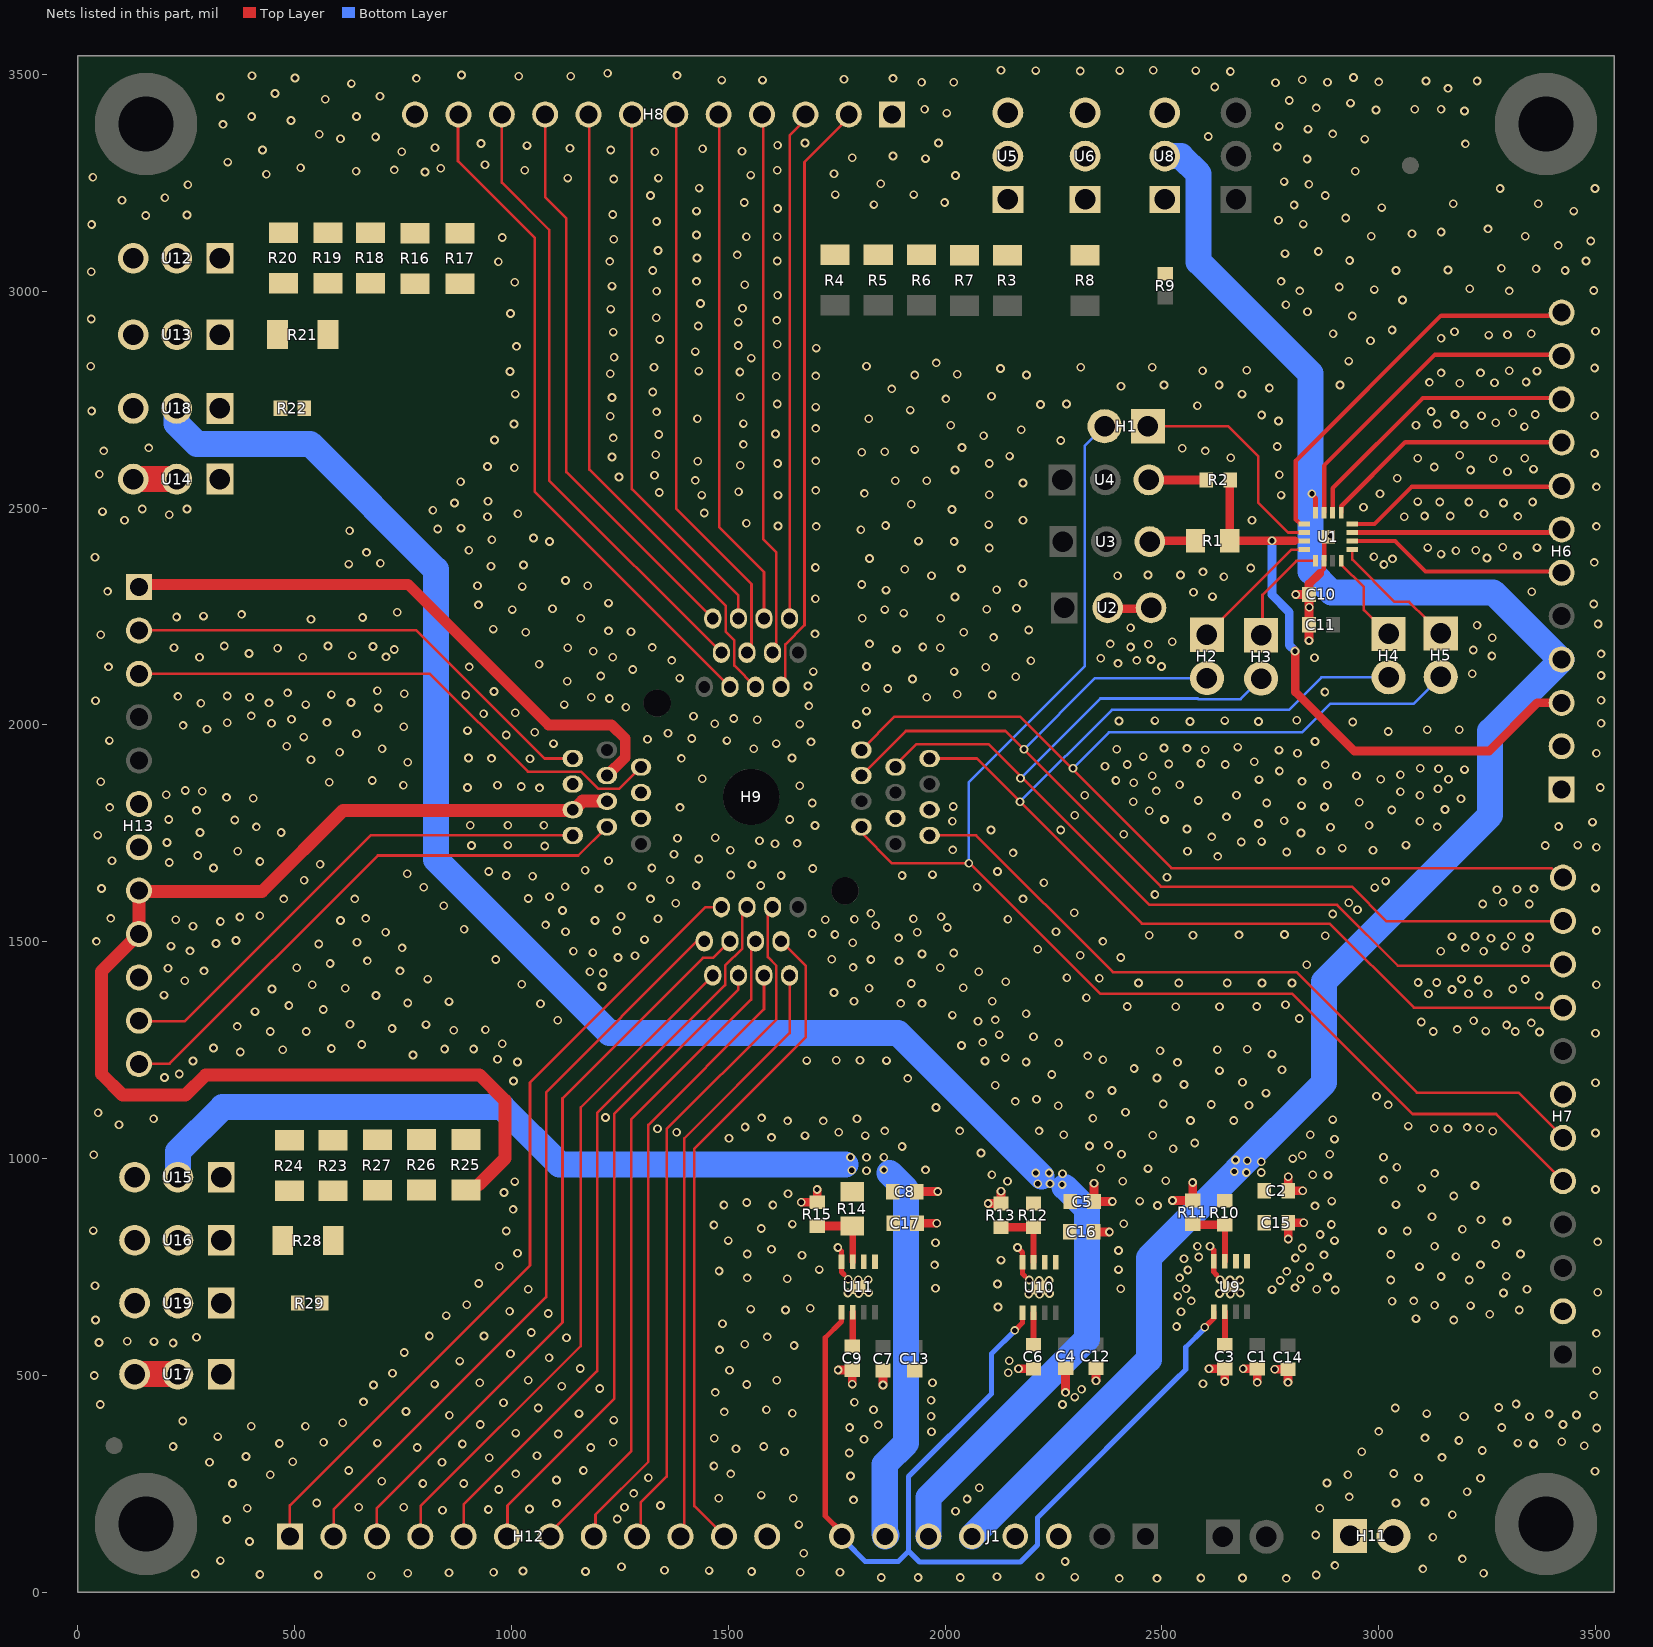
[diagram p0: the nets of this part, all layers, seen from the top]
# Altium PCB MISC79022.pcbdoc (part 2 of 3)
Units mil, origin at the board's own origin, x right, y up, seen from the top; angles counter-clockwise.
Board outline 3543.31 x 3543.31 mil, 2 copper layers (Top Layer, Bottom Layer); 79 components, 75 nets, 320 pads, 1402 vias.

## Via types
v1: diameter 20, hole 12, Top Layer to Bottom Layer, 1402 vias

## Nets (pads, with @x,y where several pads share a name; then routed paths per layer and width w, separated by ;. In a path a pad name is that pad's centre, name@x,y a point inside that pad or via, vN(x,y) a via of type N, cw(c..) or ccw(c..) an arc to the next point about the centre after c; other vN are vias at no path point) (continued)
AVSS: C1.2 C2.1 C3.1 C4.2 C5.1 C6.1 C7.2 C8.1 C9.1 C10.2 C11.1 C12.1 C13.1 C14.1 C15.1 C16.1 C17.1 H6.1 H6.2 H7.2 H7.7 H8.1 H8.12 H9.17 H9.18 H9.21 H9.40 H9.41 H11.1 H11.2 H12.12 H13.6 H13.7 H13.10 J1.3 J1.4 R11.1 R13.1 R15.1 U1.6 U1.17 U9.4 U9.9 U10.4 U10.9 U11.4 U11.9 | length 1453.3
  Top Layer w10: 2863.75,2349.75 2873.56,2359.55 2873.56,2377.98 U1.6@2874.16,2378.59 2874.16,2417.16
  Top Layer w12: v1(1753,795) 1761.6,786.4 U11.4@1761.6,762.1 1761.6,738.4 1767,733 ; v1(2167,795) 2178.6,783.4 U10.4@2178.6,761.1 2178.6,734.4 2183,730 ; v1(2611,798) 2619.55,789.45 U9.4@2619.55,763.1 2619.55,738.45 2626,732
  Top Layer w20: v1(1668.45,899.55) R15.1@1705,899.55 v1(1705,929) ; v1(1753.45,512.44) C9.1@1786,512.44 v1(1786,480) ; v1(1857,478) C7.2@1857,511.44 ; C8.1@1934.55,924 1970,924 v1(1983,924) ; C17.1@1935.55,851 v1(1981,851) ; v1(2099.45,896.55) R13.1@2129,896.55 v1(2129,925) ; v1(2169.55,515.44) C6.1@2204,515.44 ; v1(2278,461) C4.2@2278,516.44 ; C16.1@2342.55,831 v1(2379,831) ; v1(2343.55,943.44) C5.1@2343.55,901 v1(2386,901) ; v1(2348,488) C12.1@2348,516.44 ; v1(2524.55,903.55) R11.1@2571,903.55 v1(2571,945) ; v1(2608.56,515.44) C3.1@2645,515.44 v1(2645,486) ; v1(2687.44,515.44) C1.2@2720,515.44 v1(2720,484) ; v1(2760.44,514.44) C14.1@2791,514.44 v1(2791,484) ; v1(2791.56,814.55) C15.1@2791.56,852 v1(2827,852) ; v1(2791.56,958.44) C2.1@2791.56,926 v1(2825,926) ; v1(2809,2301) C10.2@2839.49,2301 ; v1(2839.44,2194.55) C11.1@2839.44,2231 v1@2839.44,2272 ; v1(2840,2271.44) v1@2839.44,2272 ; 2864,2349.5 2839.44,2324.94 v1@2839.44,2272
  other v1: 2402,32 2489,32 2787,32 2590,33 2686,33 1853,34 1938,34 2035,34 2299,35 2120,36 2219,36 677,38 555,40 2856,40 420,41 271,42 761,44 3242,44 856,45 959,46 1666,46 1758,46 1171,48 1554,48 1027,49 1456,50 1353,51 3102,54 1254,59 2899,62 2277,71 329,73 3193,77 1674,90 396,117 3125,127 2855,132 1663,156 344,168 1244,169 3170,179 2024,187 841,189 947,191 1042,192 391,194 2864,194 648,196 752,196 1261,196 1344,200 1104,205 551,206 3040,206 3107,208 1789,213 2051,215 1478,217 1650,217 2932,220 1576,224 1282,228 3204,232 971,237 2079,241 357,251 796,251 890,251 2881,252 701,256 1104,259 3235,263 1316,264 3092,264 1782,268 444,271 2929,271 1010,273 1506,273 3035,274 3499,279 625,281 1166,281 1467,291 304,300 840,300 496,301 949,310 3146,311 388,313 1059,315 1779,321 1630,324 2961,324 3239,327 1518,331 783,334 1183,334 220,336 1582,336 3474,338 887,342 3357,342 465,343 691,344 3321,344 567,346 1235,346 3422,347 3185,350 1813,353 1468,355 3107,356 323,359 1108,365 1010,367 1969,370 3000,371 3503,379 1780,380 3284,380 400,383 525,383 1846,386 928,387 3425,387 611,391 242,395 1236,397 3198,405 3348,405 1968,406 3196,406 857,408 3456,409 3393,411 1156,412 3111,412 1648,413 1491,416 757,417 1588,421 1835,421 1062,425 3038,425 3277,426 52,433 2271,433 3317,434 982,437 1791,438 659,439 1968,443 2299,450 3496,454 1470,461 2315,468 1204,470 1116,475 682,478 1543,479 823,480 2595,481 927,483 1971,483 1039,489 1612,489 38,500 726,505 2146,506 3503,511 1503,512 1159,516 881,533 2148,534 1087,541 998,550 753,553 1480,559 1652,569 1538,572 220,575 49,576 176,578 114,579 1127,587 274,588 1590,589 811,591 937,591 3502,597 1046,599 2534,613 1487,619 41,628 3173,628 3086,631 850,638 3256,641 1085,643 2544,647 996,648 1632,651 3324,651 1552,653 1689,655 2122,658 3212,661 3129,662 897,663 3031,671 2568,672 3081,672 2537,683 2218,687 2193,688 2658,688 1801,689 2241,689 2633,689 1776,690 2681,690 3288,690 1824,691 3505,692 2900,697 2754,698 1039,699 2857,699 3342,699 2405,700 2556,700 1978,701 2807,702 40,707 2121,711 925,712 2217,719 2240,719 2773,719 2194,720 2657,720 2680,720 3028,720 3209,720 1800,721 1823,721 2634,721 1777,722 2820,722 1636,723 1544,725 2541,725 2882,727 3144,728 3294,729 2788,740 1479,741 2560,743 1710,744 2400,744 2841,750 3094,751 972,752 1976,755 3235,755 2129,766 2551,769 2808,771 2585,773 3178,774 1670,777 2874,778 3028,779 1544,780 3327,780 1014,782 2400,788 1600,791 2824,794 2582,798 3129,798 3270,802 1978,806 3505,808 1500,811 2898,811 2865,825 988,833 3066,833 36,834 3009,834 3193,837 1576,839 1467,847 2891,848 1648,849 2412,850 3296,856 3236,859 3123,866 1004,883 2853,891 2490,892 1490,893 1603,893 3040,894 1543,899 2449,902 2892,902 3173,914 1638,919 983,922 3500,929 3099,932 3222,938 1008,947 2144,948 2410,948 2509,949 3012,951 2883,962 2108,963 2848,963 3129,966 1955,974 2468,977 2359,978 3042,980 2802,1000 3011,1003 2824,1008 37,1009 2407,1010 2887,1010 2083,1013 2526,1023 1901,1028 2333,1029 2377,1031 2576,1036 2898,1045 1502,1047 1600,1049 1677,1053 1816,1053 2479,1054 2274,1055 2842,1055 3500,1059 1381,1061 1755,1061 3263,1063 1861,1064 2034,1064 2217,1064 1337,1069 3160,1069 3128,1070 3233,1070 3204,1072 1539,1073 3068,1075 95,1078 1637,1087 1719,1087 2566,1088 2666,1088 2894,1090 175,1092 1797,1092 2341,1093 1577,1094 1217,1095 47,1106 2416,1107 1979,1118 2261,1122 2701,1123 3022,1124 2614,1125 2503,1126 2162,1132 2211,1137 2995,1144 2334,1147 2740,1151 2385,1157 2116,1169 2551,1171 3500,1175 2686,1176 1005,1179 1914,1185 2489,1186 200,1187 2246,1194 234,1195 2633,1203 2777,1205 2436,1208 2536,1222 1014,1223 2187,1223 266,1225 2092,1225 1681,1226 1865,1226 1749,1227 1804,1227 2364,1228 968,1229 2139,1233 2329,1237 773,1239 2754,1241 375,1246 2496,1249 473,1251 2628,1251 2697,1252 846,1253 913,1253 585,1254 313,1255 2038,1261 655,1263 979,1265 2262,1267 2087,1268 2204,1281 2125,1286 3500,1289 3371,1292 444,1293 527,1293 3126,1293 3315,1293 3247,1294 867,1296 940,1297 3181,1298 725,1300 368,1305 3295,1308 803,1309 628,1310 3352,1313 3098,1315 2076,1317 3219,1318 1107,1319 2116,1320 2817,1323 2017,1331 2187,1334 409,1339 566,1344 2532,1350 2633,1350 2420,1351 2719,1351 487,1353 2785,1355 1067,1357 1898,1358 1947,1358 761,1359 856,1362 1790,1363 2109,1363 2326,1371 3370,1375 688,1376 199,1377 3115,1380 3207,1380 3252,1380 1744,1383 3169,1390 448,1391 3309,1391 617,1393 1825,1393 2042,1394 1209,1397 541,1401 3502,1401 1024,1402 1922,1404 2446,1405 2539,1405 2651,1405 2731,1405 2800,1405 3091,1406 3134,1406 2140,1408 247,1410 3230,1412 3338,1413 807,1414 3191,1414 2356,1416 2281,1417 1212,1428 1181,1431 2078,1431 291,1433 743,1433 208,1439 505,1440 1989,1440 1788,1441 2834,1447 582,1450 668,1456 1894,1456 964,1459 1829,1459 1739,1460 1246,1464 2405,1464 1285,1468 2312,1469 1947,1472 2020,1474 1188,1475 1143,1478 3143,1478 3242,1478 259,1479 2214,1483 3340,1484 748,1486 3200,1486 215,1490 3291,1490 556,1495 319,1496 1787,1498 644,1499 43,1501 2364,1501 365,1503 1307,1505 3259,1508 1893,1509 3348,1511 3169,1512 3222,1513 3306,1513 2877,1514 2471,1515 2572,1515 2678,1516 1746,1517 2783,1517 1694,1519 710,1522 1936,1522 1125,1523 2256,1523 1243,1526 3502,1526 891,1529 2005,1533 266,1536 1840,1538 1079,1539 329,1547 606,1549 1193,1549 226,1551 1724,1551 1791,1552 2145,1552 1338,1553 1927,1553 76,1554 664,1554 374,1557 1991,1558 1253,1559 420,1560 2894,1564 1829,1566 2298,1567 1118,1572 2951,1574 844,1583 3240,1587 3347,1587 1379,1589 2931,1590 3287,1591 475,1599 639,1599 1321,1599 2180,1599 1039,1600 1088,1604 2484,1609 3273,1620 3319,1621 1202,1622 3358,1622 55,1623 3500,1624 2991,1625 798,1626 2074,1626 1124,1627 1278,1628 1426,1630 1575,1630 2228,1636 3016,1640 522,1642 1366,1643 2512,1649 1049,1651 988,1653 1622,1653 1901,1653 1506,1654 1971,1655 760,1657 948,1662 2121,1662 1170,1665 1695,1669 313,1670 1324,1670 1555,1678 559,1679 211,1683 420,1685 79,1687 1224,1687 1432,1691 2629,1697 277,1699 1375,1702 2157,1705 2788,1707 369,1709 2559,1709 2867,1710 1505,1711 2987,1711 2018,1712 2916,1716 3502,1718 1077,1721 908,1722 3384,1722 992,1723 3063,1723 3459,1723 1608,1726 1659,1727 206,1729 2683,1730 2730,1731 1572,1733 1383,1739 1470,1740 2615,1742 46,1746 2412,1748 2821,1751 282,1752 469,1752 2106,1758 2267,1758 2558,1760 2889,1764 412,1765 3135,1765 3415,1766 1700,1768 905,1769 992,1769 1075,1769 2978,1769 2723,1773 3493,1776 2017,1778 3095,1778 2782,1779 362,1781 210,1782 1642,1782 2506,1782 2649,1788 2299,1792 2471,1802 274,1803 3030,1804 3153,1805 74,1810 1389,1810 2875,1811 2019,1812 2822,1814 1694,1820 2742,1820 2955,1822 2434,1823 2584,1826 3190,1830 405,1831 343,1833 2322,1838 2672,1838 3095,1838 204,1839 3050,1846 287,1847 2487,1848 248,1849 3137,1853 1065,1855 899,1856 3511,1856 1023,1858 1665,1860 751,1861 968,1861 2882,1861 2541,1862 2435,1867 580,1868 53,1869 2823,1870 679,1872 2394,1872 2724,1874 3005,1875 3161,1875 1440,1876 2478,1883 2949,1883 3050,1885 2771,1894 3198,1897 3138,1899 3096,1900 2369,1905 2877,1908 2420,1909 2646,1909 2516,1910 2590,1911 761,1914 2713,1915 538,1920 1043,1922 954,1923 1392,1923 901,1924 1647,1924 2457,1927 2813,1935 3502,1935 604,1937 2770,1942 2600,1943 2396,1944 702,1945 1559,1945 2558,1946 2505,1947 2675,1949 482,1951 1097,1957 1611,1957 1691,1961 2853,1962 73,1964 1497,1964 1314,1967 1416,1969 521,1972 988,1977 643,1980 1361,1981 1054,1983 3022,1985 899,1987 3112,1989 3186,1989 298,1990 752,1996 243,1999 1796,2001 1665,2002 1469,2003 447,2004 3513,2004 345,2005 575,2006 2940,2007 2565,2008 2723,2008 2401,2009 2484,2010 2645,2010 2811,2011 1567,2012 493,2013 1513,2015 1420,2020 400,2021 936,2026 1009,2028 1819,2032 693,2039 1264,2041 1686,2044 526,2047 1122,2047 284,2050 441,2051 630,2052 41,2056 3513,2057 1226,2061 396,2064 1184,2064 1958,2064 231,2066 345,2067 895,2069 2109,2069 585,2070 2028,2071 753,2072 484,2074 2876,2076 960,2077 691,2079 1868,2084 1816,2086 1684,2090 1129,2101 1925,2106 1388,2108 2163,2111 1206,2113 3513,2114 3216,2118 1696,2123 2021,2123 1280,2128 2094,2133 71,2134 903,2134 1819,2135 2499,2135 1064,2140 2399,2142 2198,2148 1370,2149 2442,2149 2475,2151 2359,2154 2852,2155 281,2156 519,2156 1234,2156 711,2157 3261,2159 633,2160 3513,2164 395,2165 1189,2170 3218,2173 730,2174 1888,2175 461,2177 222,2178 1130,2178 1989,2178 1325,2179 1949,2180 2428,2180 681,2181 338,2182 577,2182 2469,2186 1826,2187 2381,2187 2524,2192 3262,2201 2112,2202 53,2208 1700,2210 1033,2214 2043,2214 1276,2215 1224,2217 2193,2219 958,2221 2428,2224 3227,2230 3506,2233 538,2244 1160,2246 1809,2246 1990,2246 657,2248 228,2249 290,2251 378,2255 1905,2258 737,2260 1002,2266 1861,2266 2096,2267 1095,2268 2165,2269 924,2277 3496,2279 1224,2281 1701,2291 2023,2295 2617,2296 2573,2306 3353,2307 69,2308 1864,2311 2119,2312 1025,2319 922,2321 1176,2321 1808,2324 2180,2327 1125,2333 2643,2342 1969,2344 2398,2344 2468,2346 2543,2346 2595,2353 1907,2359 2038,2360 2705,2362 1701,2363 953,2366 1028,2369 3012,2370 625,2371 698,2373 3497,2375 3032,2383 1826,2384 3250,2385 40,2387 2989,2388 3320,2390 3144,2394 666,2398 3178,2402 902,2403 3224,2403 2102,2408 3113,2409 3365,2409 3286,2410 1088,2423 2021,2423 1939,2424 955,2427 1051,2431 2889,2436 627,2448 1806,2450 830,2452 884,2454 1703,2458 3502,2458 1615,2459 1863,2460 2101,2462 1542,2465 108,2472 2180,2472 2708,2472 945,2480 3059,2480 3321,2481 3106,2482 3165,2482 211,2485 1015,2487 3243,2487 1445,2489 57,2492 819,2495 2016,2497 149,2498 252,2498 2965,2502 1922,2509 869,2512 3288,2512 3141,2514 3208,2514 3355,2514 3090,2515 946,2516 1439,2530 1615,2530 2775,2530 2102,2531 3003,2533 1814,2534 1341,2536 1524,2538 1702,2541 3502,2549 2180,2558 883,2561 1885,2563 1958,2563 1424,2564 3043,2569 1248,2572 1330,2576 2771,2577 50,2578 3297,2584 2023,2588 3212,2588 3357,2590 1007,2593 3128,2595 945,2596 1528,2599 1614,2603 2102,2603 1430,2608 1702,2609 3264,2614 3090,2615 3337,2615 2659,2616 1232,2618 2149,2620 3187,2622 1333,2623 3498,2626 1808,2629 1861,2630 60,2632 2600,2632 1930,2635 2547,2638 164,2639 2039,2640 2766,2642 1535,2647 2267,2656 961,2657 1235,2662 2089,2667 1340,2670 1609,2671 2176,2681 1702,2684 3336,2688 2013,2691 3086,2691 3197,2692 1006,2694 3135,2694 1535,2695 3270,2697 2769,2701 1429,2706 1824,2706 1228,2712 3237,2713 3498,2713 2730,2715 3176,2716 3361,2716 3309,2720 1335,2722 3121,2723 32,2724 1920,2726 1702,2733 2582,2736 2220,2739 1613,2740 2280,2740 2002,2752 1232,2755 1528,2757 2107,2758 1009,2763 2685,2763 1326,2768 1877,2775 2748,2777 2406,2781 2505,2784 2632,2784 2911,2784 3187,2788 3267,2789 3117,2790 3340,2791 1611,2804 1702,2805 1930,2807 2188,2807 2028,2809 1228,2810 3144,2812 3235,2812 1527,2814 997,2815 1432,2816 3365,2816 2594,2817 3301,2817 2696,2818 2128,2822 3498,2823 1329,2825 2313,2825 2478,2825 30,2827 1819,2827 1980,2835 2931,2839 1553,2846 1237,2848 1424,2861 1703,2869 1012,2873 1523,2875 1613,2878 2981,2886 1342,2889 3144,2892 3254,2899 3297,2900 2895,2902 3352,2902 1235,2906 3175,2907 3500,2908 3031,2911 1431,2920 1523,2929 1612,2933 31,2936 1334,2939 2939,2943 998,2949 2836,2953 1229,2959 1533,2961 2786,2969 1436,2972 3055,2980 1614,2991 1335,3000 2818,3001 3301,3001 3496,3002 2990,3004 3210,3006 2909,3010 1232,3012 1538,3015 1008,3021 1427,3023 2775,3023 31,3045 1326,3048 3040,3048 3430,3048 3160,3049 3363,3052 3283,3053 970,3068 1227,3069 1613,3070 3478,3070 2933,3071 1428,3077 1521,3084 2784,3087 2861,3092 1338,3094 3414,3106 3489,3116 1236,3120 979,3124 1542,3126 1613,3126 2983,3127 3338,3127 1427,3130 3077,3133 3144,3137 3252,3144 32,3154 2826,3155 1335,3161 2769,3164 2924,3169 157,3175 252,3176 1234,3177 1427,3185 3450,3185 1614,3191 3007,3193 2805,3199 1836,3200 3172,3202 3368,3202 1537,3205 1999,3205 102,3210 201,3216 1321,3221 2877,3221 1747,3223 1928,3223 3280,3237 3499,3237 1433,3238 254,3246 2839,3247 1852,3248 2782,3253 1236,3259 1130,3261 1339,3261 35,3263 2024,3267 1552,3268 435,3270 1744,3271 801,3275 642,3277 2946,3277 1031,3279 1613,3279 730,3280 837,3284 514,3285 939,3292 346,3298 2835,3305 1955,3306 1786,3308 1880,3312 747,3322 1331,3322 1532,3323 426,3326 1229,3326 1441,3329 1135,3330 824,3331 2766,3333 1036,3336 1614,3337 3200,3340 930,3341 1677,3342 1985,3342 2968,3351 606,3352 687,3356 2607,3357 557,3362 2894,3363 2837,3374 2771,3381 335,3385 492,3394 401,3403 643,3403 2004,3411 3198,3416 2994,3418 1953,3420 3083,3420 3144,3420 2856,3423 2935,3434 2794,3440 571,3443 329,3448 697,3450 455,3456 3160,3468 2622,3471 631,3479 2762,3481 1946,3482 2020,3482 2882,3482 3000,3483 3109,3485 3227,3485 1485,3487 1579,3487 2824,3488 1767,3489 781,3491 1880,3491 501,3492 2942,3493 1017,3496 1137,3496 402,3497 1382,3498 885,3499 1222,3503 2658,3507 2312,3508 2209,3509 2403,3509 2578,3509 2129,3510 2480,3510
CUR_IN: U2.2 U2.3 | length 95.8
  Top Layer w20: U2.2@2375,2270 2377,2268 U2.3@2470,2268
DAC_ADC_IN: H6.3 R1.2 R2.2 U1.3 | length 1411
  Top Layer w10: 2806.36,2424.16 U1.3@2828.59,2424.16
  Top Layer w20: 2656.37,2510.37 2656.37,2493 ; R2.2@2656.37,2556.63 2656.37,2493 ; 2806.36,2424.84 2656.53,2424.84 R1.2@2656.37,2425 2656.37,2493 ; v1(2807,2170) 2808,2171 2808,2076 2944,1940 3255,1940 3366,2051 H6.3@3422,2051
  Bottom Layer w20: v1(2754,2425) 2754,2300 2794,2260 2794,2184 2807,2171 v1(2807,2170)
DAC_CLK: H6.9 U1.13 | length 572.7
  Top Layer w10: U1.13@2913.53,2489.41 2913.53,2504.53 3061,2652 H6.9@3410,2652
DAC_DATA_OUT: H6.11 U1.15 | length 750.6
  Top Layer w10: U1.15@2874.16,2489.41 2874.16,2598.16 3130,2854 H6.11@3410,2854
DAC_EN: H6.8 U1.12 | length 513
  Top Layer w10: U1.12@2939.41,2463.53 2990.53,2463.53 3076,2549 H6.8@3417,2549
DAC_HEAD: H1.1 U1.2 | length 502.8
  Top Layer w6: H1.1@2490,2689 2546,2689 2653,2689 2722,2620 2722,2513 2791.16,2443.84 U1.2@2828.59,2443.84
DAC_IN: H6.10 U1.14 | length 660.8
  Top Layer w10: U1.14@2893.84,2489.41 2893.84,2545.84 3102,2754 H6.10@3412,2754
DAC_OTA_BIAS: H5.1 U1.9 | length 250.5
  Top Layer w6: U1.9@2939.41,2404.47 2939.41,2381.59 3037,2284 3070,2284 H5.1@3110,2244
DAC_OUT6: H6.6 U1.10 | length 565.6
  Top Layer w10: U1.10@2939.41,2424.16 3037.84,2424.16 3108,2354 3303,2354 ; 3364,2354 3303,2354 ; H6.6@3415,2354 3303,2354
DAC_OUT7: H6.7 U1.11 | length 584.9
  Top Layer w11: U1.11@2939.41,2443.84 3249,2443.84 ; 3371.16,2443.84 3249,2443.84 ; H6.7@3402.16,2443.84 3249,2443.84
DAC_REF_OUT: H6.12 U1.1 | length 910.7
  Top Layer w10: U1.1@2828.59,2463.53 2819.47,2463.53 2809,2474 2809,2609 3144,2944 H6.12@3422,2944
DAC_VBIASN: H4.1 U1.8 | length 167.8
  Top Layer w6: U1.8@2913.53,2378.59 2913.53,2370.47 2966,2318 2966,2265 H4.1@2989,2242
DAC_VBIASP: H3.1 U1.5 | length 216
  Top Layer w6: H3.1@2732,2239 2732,2300 2810.59,2378.59 U1.5@2854.47,2378.59
DAC_VCLAMP: H2.1 U1.4 | length 268.8
  Top Layer w6: H2.1@2630,2235 2799.47,2404.47 U1.4@2828.59,2404.47
DSIGN: H9.14 H13.2 | length 1108.9
  Top Layer w6: H13.2@155,2218 198,2218 781,2218 1076.42,1922.58 H9.14@1141.58,1922.58
DVDD: H9.19 H9.20 H13.8 H13.9 R23.2 R24.2 R25.2 R26.2 R27.2 R28.2 R29.2 U17.1 | length 2810
  Top Layer w30: H13.9@141,1518 55,1432 55,1195 103,1147 249,1147 295,1193 927,1193 985,1135 985,1000 R25.2@925,940 ; H13.9@141,1534 H13.8@141,1618 ; H13.8@152,1616 425,1616 612,1803 1143,1803 1164.16,1824.16 H9.19@1220.32,1824.16
DVDD_CUR_IN: U17.2 U17.3 | length 103
  Top Layer w60: U17.3@128,503 U17.3@131,503 U17.2@231,503
DVDDIO: H9.16 H13.1 R16.2 R17.2 R18.2 R19.2 R20.2 R21.2 R22.2 U14.1 | length 1356.5
  Top Layer w25: H13.1@156,2324 762,2324 1086,2000 1231,2000 1262.44,1968.56 1262.44,1925.33 H9.16@1220.32,1883.21
DVDDIO_CUR_IN: U14.2 U14.3 | length 100
  Top Layer w60: U14.3@128,2567 U14.2@228,2567
EN_LDO: J1.8 U9.5 U10.5 U11.5 | length 2416.2
  Top Layer w12: J1.8@1761,139 1724,176 1724,587 1761.6,624.6 U11.5@1761.6,645.9 ; v1(2161,604) 2178.6,621.6 U10.5@2178.6,644.9 ; v1@2604,616 2619.55,631.55 U9.5@2619.55,646.9
  Bottom Layer w12: J1.8@1769,118 1816,71 1892,71 1914,93 ; v1(2161,604) 2107,550 2107,458 1916,267 1916,95 1941,70 2174,70 2213,109 2213,172 2529,488 ; 2548,507 2529,488 ; v1@2598,608 2555,565 2555,514 2529,488
  other v1: 2599,611
HEAD: H1.2 H7.5 H9.39 | length 3087.2
  Top Layer w6: H9.39@1806.94,1765.1 1806.94,1752.06 1878,1681 2058,1681 2359,1380 2801,1380 3078,1103 3271,1103 H7.5@3415,959
  Bottom Layer w6: v1(2055,1681) 2055,1868 2322,2135 2322,2643 H1.2@2368,2689
LDO_AVDD: C2.2 C15.2 H6.4 J1.5 R10.1 U1.16 U5.2 U5.3 U6.2 U6.3 U8.2 U8.3 U9.1 U9.2 | length 4415.7
  Top Layer w11: v1@2847,2530 2854.47,2522.53 U1.16@2854.47,2489.41
  Bottom Layer w60: J1.5@2062,129 2470,537 2470,722 2470,771 2675,976 ; U8.2@2507,3312 2544,3312 2585,3271 2585,3068 2843,2810 2843,2354 2891,2306 3264,2306 H6.4@3420.5,2149.5 ; v1@2671,972 2874,1175 2874,1409 3257,1792 3257,1986 H6.4@3420.5,2149.5 ; H6.4@3422,2151 H6.4@3420.5,2149.5
  other v1: 2695,968 2729,968 2667,970 2729,993 2697,995 2670,997 2846,2533
LDO_DVDD: C8.2 C17.2 J1.7 R14.1 U11.1 U11.2 U15.2 U15.3 U16.2 U16.3 U19.2 U19.3 | length 2569
  Bottom Layer w60: U15.2@231,957 231,1016 334,1119 979,1119 ; 978,1120 979,1119 ; 1771,987 1241,987 1111,987 979,1119 ; J1.7@1861,136 1861,295 1910,344 1910,929 1872,967 ; J1.7@1862,129 J1.7@1865,132
  other v1: 1819,972 1785,973 1859,974 1782,1003 1819,1003 1859,1003
LDO_DVDDIO: C5.2 C16.2 J1.6 R12.1 U10.1 U10.2 U12.2 U12.3 U13.2 U13.3 U18.2 U18.3 | length 4117.7
  Bottom Layer w60: U18.2@228,2730 228,2695 275,2648 536,2648 826,2358 826,1690 1226,1290 1891,1290 2222,959 ; J1.6@1962,129 1962,219 2327,584 2327,884 v1@2276,935
  other v1: 2270,940 2214,942 2242,942 2271,965 2209,967 2240,967
NEG0: H8.9 H9.11 | length 1350.6
  Top Layer w6: 1078,3366 1078,3328 ; H8.9@1078,3398 1078,3328 ; H9.11@1464.42,2245.42 1127,2582.83 1127,3168 1078,3217 1078,3328
NEG1: H8.10 H9.10 | length 1441
  Top Layer w6: H8.10@978,3398 978,3251 1087,3142 1087,2563.78 H9.10@1484.1,2166.68
NEG2: H8.11 H9.9 | length 1573.7
  Top Layer w6: H8.11@877,3402 877,3300 1054,3123 1054,2537.72 H9.9@1503.79,2087.94
NEG3: H8.7 H9.8 | length 1363.3
  Top Layer w6: 1278,3368 1278,3263 ; H8.7@1278,3402 1278,3263 ; H9.8@1523.47,2245.42 1523.47,2298.53 1278,2544 1278,3263
NEG4: H8.6 H9.7 | length 1363.8
  Top Layer w6: 1380,3369 1380,3324 ; H8.6@1380,3409 1380,3324 ; H9.7@1543.16,2166.68 1553.84,2177.36 1553.84,2325.16 1380,2499 1380,3324
NEG5: H8.8 H9.6 | length 1492.6
  Top Layer w6: 1180,3363 1180,3336 ; H8.8@1180,3395 1180,3336 ; H9.6@1562.84,2087.94 1514,2136.78 1514,2195 1494,2215 1494,2275 1180,2589 1180,3336
NEG6: H8.5 H9.5 | length 1178.5
  Top Layer w6: H8.5@1479,3381 1479,2456 1582.53,2352.47 H9.5@1582.53,2245.42
NEG7: H8.4 H9.4 | length 1241.6
  Top Layer w6: H8.4@1581,3392 1581,2428 1611.21,2397.79 1611.21,2175.68 H9.4@1602.21,2166.68
NEG8: H8.2 H9.3 | length 1388
  Top Layer w6: H9.3@1621.9,2087.94 1632,2098.04 1632,2186 1676,2230 1676,3202 1676,3298 H8.2@1786,3408
NEG9: H8.3 H9.2 | length 1160
  Top Layer w6: H9.2@1641.58,2245.42 1641.58,3359.58 H8.3@1674,3392
NetC3_2: C3.2 U9.6 | length 72.1
  Top Layer w14: C3.2@2645.15,574.85 U9.6@2645.15,646.9
NetC6_2: C6.2 U10.6 | length 67.7
  Top Layer w14: C6.2@2204.2,577.2 U10.6@2204.2,644.9
NetC9_2: C9.2 U11.6 | length 72.7
  Top Layer w14: C9.2@1787.2,573.2 U11.6@1787.2,645.9
NetR1_1: R1.1 U3.3 | length 103.6
  Top Layer w20: U3.3@2474,2425 R1.1@2577.63,2425
NetR2_1: R2.1 U4.3 | length 119.4
  Top Layer w20: U4.3@2483,2565 2534,2565 R2.1@2602.44,2565
NetR3_1: R3.1 R4.1 R5.1 R6.1 R7.1 U5.1
NetR8_1: R8.1 U6.1
NetR9_1: R9.1 U8.1
NetR10_2: R10.2 R11.2 U9.3 | length 152.6
  Top Layer w14: U9.3@2645.15,763.1 R10.2@2645.15,841.15
  Top Layer w20: R11.2@2570.45,847.44 R10.2@2645,847.44
NetR12_2: R12.2 R13.2 U10.3 | length 141.3
  Top Layer w14: U10.3@2204.2,761.1 R12.2@2204.2,831.8
  Top Layer w20: R13.2@2133.45,841.44 R12.2@2204,841.44
NetR14_2: R14.2 R15.2 U11.3 | length 144.3
  Top Layer w14: U11.3@1787.2,762.1 R14.2@1787.2,830.8
  Top Layer w20: R15.2@1710.37,844.63 R14.2@1786,844.63
NetR16_1: R16.1 R17.1 R18.1 R19.1 R20.1 U12.1
NetR21_1: R21.1 U13.1
NetR22_1: R22.1 U18.1
NetR23_1: R23.1 R24.1 R25.1 R26.1 R27.1 U15.1
NetR28_1: R28.1 U16.1
NetR29_1: R29.1 U19.1
OTA_BIAS: H5.2 H7.12 H9.48 | length 2726.4
  Top Layer w6: H9.48@1806.94,1942.27 1883.67,2019 2173,2019 2522,1670 3399,1670 H7.12@3415,1654
  Bottom Layer w6: v1(2295,1900) 2378,1983 2823,1983 2889,2049 3081,2049 H5.2@3143,2111
POS0: H9.35 H12.10 | length 1384.1
  Top Layer w6: H12.10@1399,139 1399,1047 1641.58,1289.58 H9.35@1641.58,1422.58
POS1: H9.34 H12.11 | length 1515.9
  Top Layer w6: H12.11@1481,140 1422,199 1422,1023 1679,1280 1679,1444.22 H9.34@1621.9,1501.32
POS2: H9.33 H12.9 | length 1595.4
  Top Layer w6: H12.9@1298,127 1298,207 1358,267 1358,1068 1611.21,1321.21 1611.21,1444.79 1591.53,1464.47 1591.53,1569.38 H9.33@1602.21,1580.06
POS3: H9.32 H12.8 | length 1443.5
  Top Layer w6: H12.8@1194,140 1194,179 1316,301 1316,1078 1582.53,1344.53 H9.32@1582.53,1422.58
POS4: H9.31 H12.7 | length 1559.6
  Top Layer w6: H12.7@1089,138 1276,325 1276,1090 1553,1367 1553,1491.48 H9.31@1562.84,1501.32
POS5: H9.30 H12.5 | length 1721.6
  Top Layer w6: H12.5@890,129 890,202 1198,510 1198,1105 1493.1,1400.1 1493.1,1445.1 1532.47,1484.47 1532.47,1569.38 H9.30@1543.16,1580.06
POS6: H9.29 H12.6 | length 1511.1
  Top Layer w6: H12.6@991,143 991,197 ; 991,186 991,197 ; H9.29@1523.47,1422.58 1523.47,1389.47 1237,1103 1237,446 991,200 991,197
POS7: H9.28 H12.3 | length 1723.1
  Top Layer w6: H12.3@690,129 690,194 1118,622 1118,1139 1442,1463 1465.46,1463 H9.28@1503.79,1501.32
POS8: H9.27 H12.1 | length 1886.4
  Top Layer w6: H12.1@489,145 489,200 ; 489,182 489,200 ; H9.27@1484.1,1580.06 1448.06,1580.06 1043,1175 1043,754 489,200
POS9: H9.26 H12.4 | length 1572.5
  Top Layer w6: H12.4@790,129 H12.4@790,138 ; H12.4@791,138 791,199 1160,568 1160,1118.17 H9.26@1464.42,1422.58
RST: H9.15 H13.3 | length 1337.4
  Top Layer w6: H13.3@137,2125 144,2118 234,2118 ; 192,2118 234,2118 ; H9.15@1299.06,1902.9 1249.17,1853 1200,1853 1160.79,1892.21 1037.79,1892.21 812,2118 234,2118
S0: H9.25 H12.2 | length 1736
  Top Layer w6: H12.2@590,129 590,191 1080,681 1080,1153 1428.32,1501.32 H9.25@1444.73,1501.32
S1: H9.23 H13.11 | length 1169
  Top Layer w6: H13.11@150,1317 247,1317 675.42,1745.42 H9.23@1141.58,1745.42
S2: H9.22 H13.12 | length 1304.5
  Top Layer w6: H13.12@142,1219 212,1219 692,1699 1154.22,1699 H9.22@1220.32,1765.1
SAMPLE: H7.6 H9.38 | length 1732.1
  Top Layer w6: H9.38@1964.42,1745.42 2071.58,1745.42 2387,1430 2810,1430 3088,1152 3322,1152 H7.6@3413,1061
VBIASN: H4.2 H7.9 H9.47 | length 2724.5
  Top Layer w6: H9.47@1964.42,1922.58 2073.42,1922.58 2454,1542 2887,1542 3081,1348 3300,1348 ; 3372,1348 3300,1348 ; H7.9@3410,1348 3300,1348
  Bottom Layer w6: v1(2173,1823) 2385,2035 2793,2035 2868,2110 H4.2@3023,2110
VBIASP: H3.2 H7.10 H9.46 | length 2417.2
  Top Layer w6: H9.46@1885.68,1902.9 1885.68,1907.68 1934,1956 2100,1956 2471,1585 2904,1585 3044,1445 H7.10@3415,1445
  Bottom Layer w6: v1(2174,1877) 2358,2061 2582.59,2061 2583.96,2059.63 2681.63,2059.63 H3.2@2729,2107
VCLAMP: H2.2 H7.11 H9.45 | length 2393.4
  Top Layer w6: H9.45@1806.94,1883.21 1909.72,1986 2139,1986 2498,1627 2938,1627 3018,1547 3303,1547 ; 3379,1547 3303,1547 ; H7.11@3410,1547 3303,1547
  Bottom Layer w6: v1(2182,1944) 2346,2108 H2.2@2604,2108
pads on no net: H9.0 H9.1 H9.12 H9.13 H9.24 H9.36 H9.37